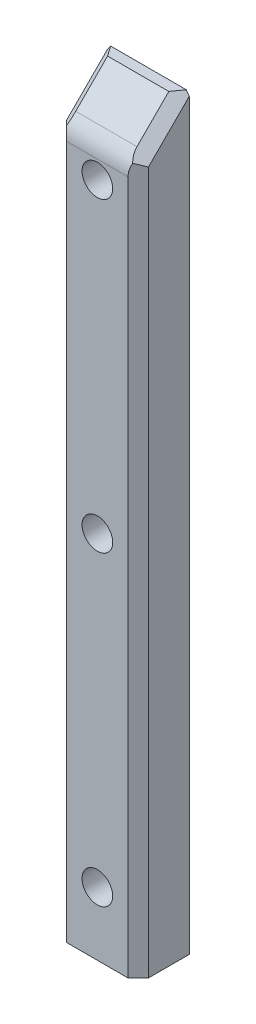
SolidWorks part; units mm, degrees
ref_plane "Front Plane" through (0, 0, 0) normal (0, 0, 1) x (1, 0, 0)
ref_plane "Top Plane" through (0, 0, 0) normal (0, 1, 0) x (1, 0, 0)
ref_plane "Right Plane" through (0, 0, 0) normal (1, 0, 0) x (0, 0, -1)
sketch "Sketch1" plane through (0, 0, 0) normal (0, 0, 1) x (1, 0, 0)
  line L1 (-20, 183) -> (20, 183)
  line L2 (-20, 183) -> (-20, -183)
  line L3 (-20, -183) -> (20, -183)
  line L4 (20, 183) -> (20, -183)
  line L5 (-20, 183) -> (20, -183) construction
  line L6 (-20, -183) -> (20, 183) construction
  point P0 (0, 0)
  dimension "D1" = 40
  dimension "D2" = 366
extrude "Boss-Extrude1" add sketch "Sketch1" along normal blind 25
chamfer "Chamfer1" [suppressed] distance 20 angle 30
hole_wizard "M6 Tapped Hole1" positions "Sketch2" profile "Sketch3" tap size "M6" standard "GB"
sketch "Sketch2" plane through (0, 0, 0) normal (0, 0, -1) x (-1, 0, 0)
  line L0 (0, 150) -> (0, 175) construction
  line L1 (-20, 175) -> (20, 175) construction
  line L6 (20, -175) -> (-20, -175) construction
  point P0 (0, 150)
  point P5 (0, -150)
  point P19 (0, 0)
  dimension "D1" = 25
  dimension "D2" = 150
  dimension "D3" = 150
sketch "Sketch3" plane through (0, 150, 0) normal (1, 0, 0) x (0, 1, 0)
  line L0 (0, 0) -> (0, 27)
  line L1 (0, 27) -> (2.5, 27)
  line L2 (2.5, 27) -> (2.5, 0)
  line L5 (2.5, 0) -> (0, 0)
  line L11 (0, -6.35) -> (0, 107.95) construction
  dimension "通孔螺纹孔钻头直径" = 5
  dimension "通孔螺纹孔钻头深度" = 27
cosmetic thread "Cosmetic Thread1" [suppressed] parameters "D2"=6
cosmetic thread "Cosmetic Thread2" [suppressed] parameters "D2"=6
cosmetic thread "Cosmetic Thread3" [suppressed] parameters "D2"=6
chamfer "Chamfer2" distance 20 angle 45 1 edges at (0, 183, 25)
sketch "Sketch4" plane through (0, 0, 25) normal (0, 0, 1) x (1, 0, 0)
  line L0 (0, -183) -> (0, -152) construction
  line L1 (-20, -183) -> (20, -183) construction
  circle A0 centre (0, -152) radius 7.5
  circle A1 centre (0, -2) radius 7.5
  circle A2 centre (0, 148) radius 7.5
  dimension "D1" = 15
  dimension "D2" = 31
  dimension "D3" = 150
  dimension "D4" = 150
extrude "Cut-Extrude1" cut sketch "Sketch4" against normal blind 2
hole_wizard "Hole Size (based on) hex socket cap screw type 1" positions "Sketch5" profile "Sketch6" counterbore size "M8" standard "GB" end condition through all
sketch "Sketch5" plane through (0, 0, 23) normal (0, 0, 1) x (1, 0, 0)
  point P0 (0, -152)
  point P3 (0, -2)
  point P6 (0, 148)
sketch "Sketch6" plane through (0, -152, 23) normal (1, 0, 0) x (0, -1, 0)
  line L0 (0, 0) -> (0, 23)
  line L1 (0, 23) -> (4.5, 23)
  line L3 (4.5, 23) -> (4.5, 10)
  line L4 (4.5, 10) -> (7.5, 10)
  line L5 (7.5, 10) -> (7.5, 0)
  line L7 (7.5, 0) -> (0, 0)
  line L11 (0, -6.35) -> (0, 107.95) construction
  dimension "通孔孔直径" = 9
  dimension "通孔孔深度" = 23
  dimension "柱形沉头孔直径" = 15
  dimension "柱形沉头孔深度" = 10
sketch "Sketch7" plane through (0, 0, 25) normal (0, 0, 1) x (1, 0, 0)
  line L0 (-20, -179) -> (15, -183)
  line L1 (-20, 163) -> (-20, -183) construction
  line L2 (-20, -183) -> (20, -183) construction
  line L3 (15, -183) -> (-20, -183)
  line L4 (-20, -183) -> (-20, -179)
  dimension "D1" = 35
  dimension "D2" = 4
extrude "Cut-Extrude2" [suppressed] cut sketch "Sketch7" against normal through all
fillet "Fillet1" [suppressed] radius 5
sketch "Sketch8" [suppressed] plane through (0, 0, 25) normal (0, 0, 1) x (1, 0, 0)
  line L0 (-15, -185) -> (20, -181)
  line L1 (-15, -185) -> (15, -185) construction
  line L2 (20, 164.0054) -> (20, -185) construction
  line L3 (20, -181) -> (20, -185)
  line L4 (20, -185) -> (-15, -185)
  dimension "D1" = 35
  dimension "D2" = 4
extrude "Cut-Extrude3" [suppressed] cut sketch "Sketch8" against normal through all
chamfer "Chamfer3" distance 5 angle 45 2 edges at (20, -10, 25) (-20, -10, 25)
fillet "Fillet2" [suppressed] radius 5
fillet "Fillet3" [suppressed] radius 10
chamfer "Chamfer4" distance 5 angle 45 2 edges at (20, 175.5, 12.5) (-20, 175.5, 12.5)
fillet "Fillet4" radius 15 1 edges at (0, 163, 25)
